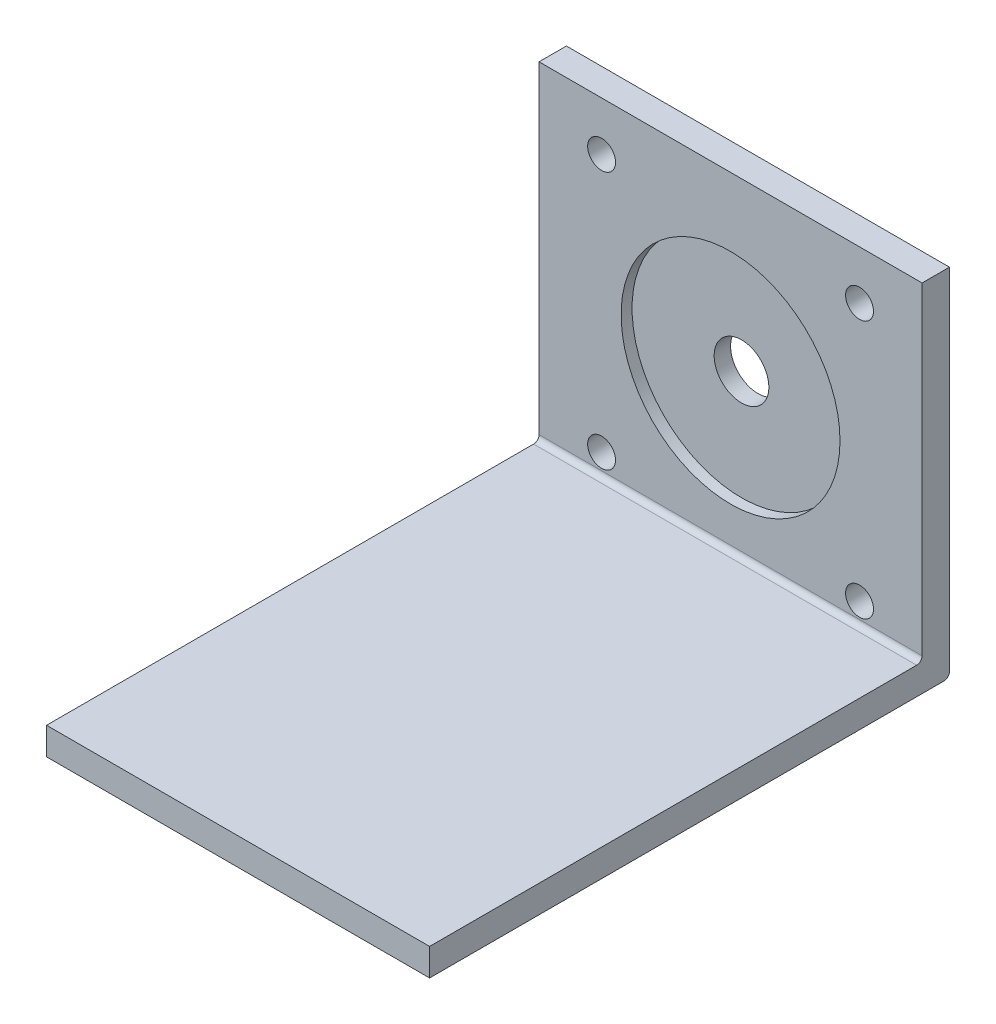
SolidWorks part; units mm, degrees
material "1060 合金"
ref_plane "前视基准面" through (0, 0, 0) normal (0, 0, 1) x (1, 0, 0)
ref_plane "上视基准面" through (0, 0, 0) normal (0, 1, 0) x (1, 0, 0)
ref_plane "右视基准面" through (0, 0, 0) normal (1, 0, 0) x (0, 0, -1)
other "Configuration Table"
sketch "草图1" plane through (0, 0, 0) normal (0, 0, 1) x (1, 0, 0)
  line L1 (-23.57, -23.57) -> (23.57, -23.57) construction
  line L2 (-23.57, -23.57) -> (-23.57, 23.57) construction
  line L3 (-23.57, 23.57) -> (23.57, 23.57) construction
  line L4 (23.57, -23.57) -> (23.57, 23.57) construction
  line L5 (-23.57, -23.57) -> (23.57, 23.57) construction
  line L6 (-23.57, 23.57) -> (23.57, -23.57) construction
  line L7 (-35, -32.5) -> (35, -32.5)
  line L8 (-35, -32.5) -> (-35, 32.5)
  line L9 (-35, 32.5) -> (35, 32.5)
  line L10 (35, -32.5) -> (35, 32.5)
  line L11 (-35, -32.5) -> (35, 32.5) construction
  line L12 (-35, 32.5) -> (35, -32.5) construction
  circle A0 centre (-23.57, 23.57) radius 2.25
  circle A1 centre (23.57, 23.57) radius 2.25
  circle A2 centre (23.57, -23.57) radius 2.25
  circle A3 centre (-23.57, -23.57) radius 2.25
  point P0 (0, 0)
  point P6 (0, 0)
  dimension "D5" = 4.5
  dimension "D1" = 47.14
  dimension "D2" = 47.14
  dimension "D3" = 65
  dimension "D4" = 70
extrude "凸台-拉伸1" add sketch "草图1" along normal blind 5 contours L8 L7 L10 L9
sketch "草图3" plane through (0, 0, 5) normal (0, 0, 1) x (1, 0, 0)
  line L1 (-23.57, -23.57) -> (23.57, -23.57) construction
  line L2 (-23.57, -23.57) -> (-23.57, 23.57) construction
  line L3 (-23.57, 23.57) -> (23.57, 23.57) construction
  line L4 (23.57, -23.57) -> (23.57, 23.57) construction
  line L5 (-23.57, -23.57) -> (23.57, 23.57) construction
  line L6 (-23.57, 23.57) -> (23.57, -23.57) construction
  line L11 (-26.0841, -23.9965) -> (26.0841, 23.9965) construction
  line L12 (-26.0841, 23.9965) -> (34.9655, -32.1671) construction
  circle A0 centre (-23.57, 23.57) radius 2.55
  circle A1 centre (23.57, 23.57) radius 2.55
  circle A2 centre (23.57, -23.57) radius 2.55
  circle A3 centre (-23.57, -23.57) radius 2.55
  point P0 (0, 0)
  point P6 (0, 0)
  dimension "D5" = 5.1
  dimension "D1" = 47.14
  dimension "D2" = 47.14
extrude "切除-拉伸2" cut sketch "草图3" against normal through all both and the other way through all
sketch "草图4" plane through (0, 0, 5) normal (0, 0, 1) x (1, 0, 0)
  line L0 (35, -32.5) -> (35, 32.5) construction
  line L1 (-35, -32.5) -> (35, -32.5)
  line L2 (-35, -32.5) -> (-35, -27.5)
  line L3 (-35, -27.5) -> (35, -27.5)
  line L4 (35, -32.5) -> (35, -27.5)
  dimension "D1" = 5
extrude "凸台-拉伸2" add sketch "草图4" along normal blind 90
fillet "圆角1" radius 1 1 edges at (0, -27.5, 5)
fillet "圆角2" radius 1 1 edges at (0, -32.5, 0)
sketch "草图5" plane through (0, 0, 0) normal (0, 0, -1) x (-1, 0, 0)
  circle A0 centre (0, 0) radius 20
  dimension "D1" = 40
extrude "切除-拉伸3" cut sketch "草图5" along normal blind 2 from surface at -5 starting at face at (0, 3, 5)
sketch "草图6" plane through (0, 0, 3) normal (0, 0, 1) x (1, 0, 0)
  circle A0 centre (0, 0) radius 5
  dimension "D1" = 10
extrude "切除-拉伸4" cut sketch "草图6" against normal through all both and the other way through all
